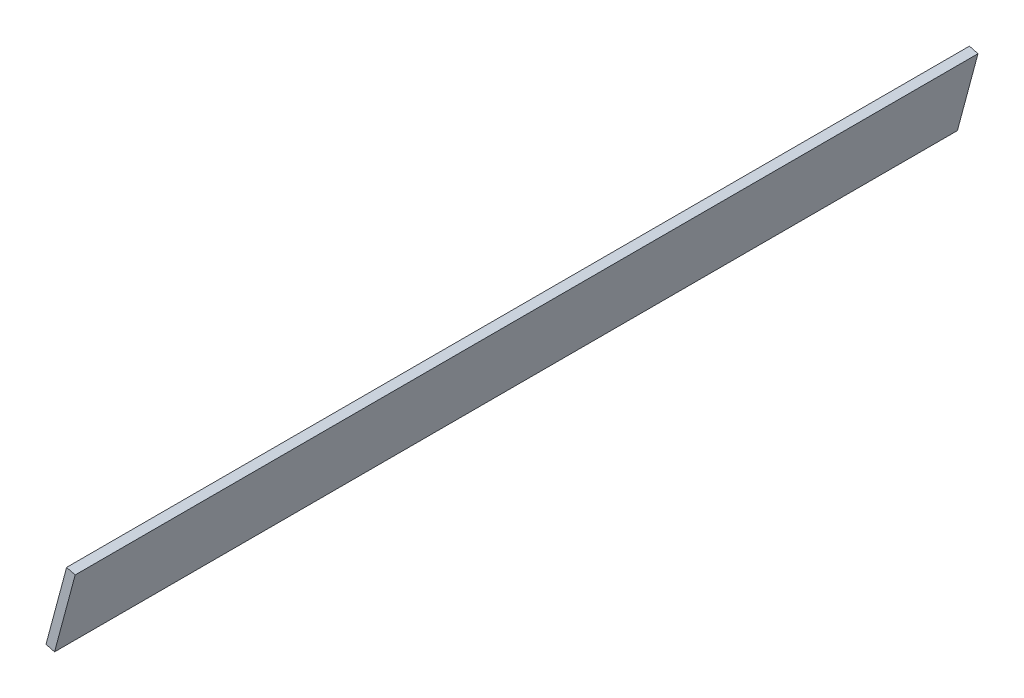
SolidWorks part; units mm, degrees
ref_plane "前视基准面" through (0, 0, 0) normal (0, 0, 1) x (1, 0, 0)
ref_plane "上视基准面" through (0, 0, 0) normal (0, 1, 0) x (1, 0, 0)
ref_plane "右视基准面" through (0, 0, 0) normal (1, 0, 0) x (0, 0, -1)
ref_plane "基准面4" through (2654.7128, -711.3281, 0) normal (-0.9659, 0.2588, 0) x (-0.2588, -0.9659, 0)
sketch "草图1" plane through (2654.7128, -711.3281, 0) normal (-0.9659, 0.2588, 0) x (-0.2588, -0.9659, 0)
  line L0 (-2157.781, 88.1446) -> (-2139.781, 88.1446)
  line L1 (-2139.781, 88.1446) -> (-2139.781, 292.1446)
  line L2 (-2139.781, 292.1446) -> (-2157.781, 292.1446)
  line L3 (-2157.781, 292.1446) -> (-2157.781, 88.1446)
extrude "凸台-拉伸1" add sketch "草图1" against normal blind 2
